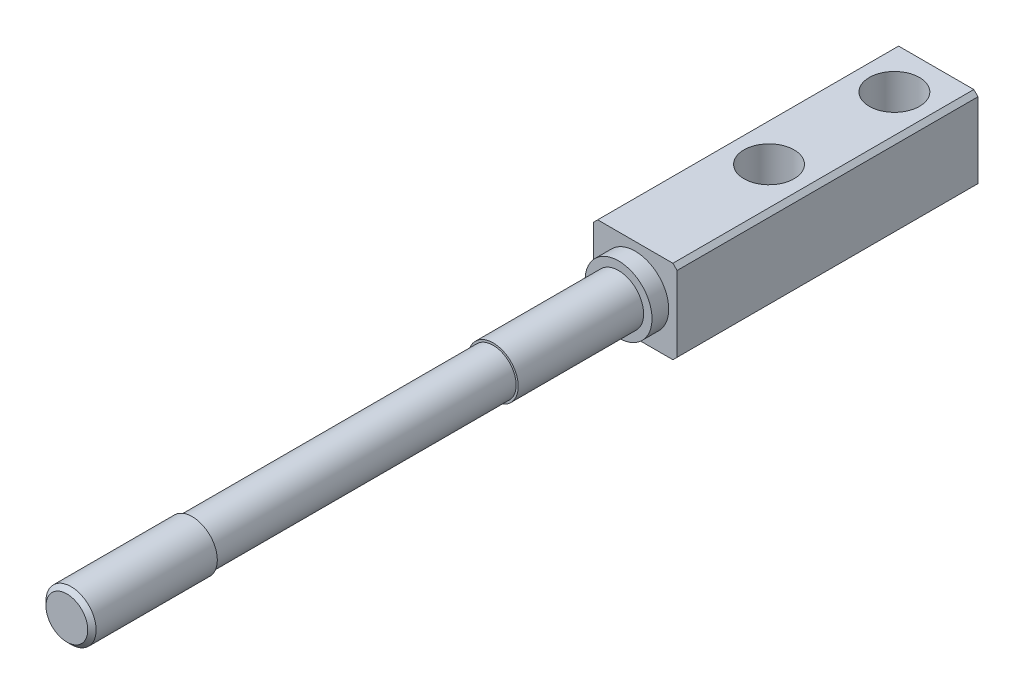
from build123d import *

# Parameters (mm, degrees)
SKETCH1_W           = 10
SKETCH1_H           = 10
BOSS_EXTRUDE1_DEPTH = 36
SKETCH2_R           = 4
BOSS_EXTRUDE2_DEPTH = 2
SKETCH3_R           = 3
BOSS_EXTRUDE3_DEPTH = 66
SKETCH4_R           = 3
CUT_EXTRUDE1_DEPTH  = 50
CHAMFER1_SIZE       = 0.5
CHAMFER2_SIZE       = 0.5
SKETCH6_W           = 5
SKETCH6_H           = 36


with BuildPart() as part:
    # Sketch1 → Boss-Extrude1 (new body)
    with BuildSketch(Plane.XY):
        Rectangle(SKETCH1_W, SKETCH1_H)
    extrude(amount=BOSS_EXTRUDE1_DEPTH)

    # Sketch2 → Boss-Extrude2 (add)
    with BuildSketch(Plane.XY.offset(36)):
        Circle(SKETCH2_R)
    extrude(amount=BOSS_EXTRUDE2_DEPTH)

    # Sketch3 → Boss-Extrude3 (add)
    with BuildSketch(Plane.XY.offset(38)):
        Circle(SKETCH3_R)
    extrude(amount=BOSS_EXTRUDE3_DEPTH)

    # Sketch4 → Cut-Extrude1 (cut)
    with BuildSketch(Plane(origin=(0, 5, 0), x_dir=(1, 0, 0), z_dir=(0, 1, 0))):
        with Locations(Location((0, -5, 0), (0, 0, 270))):
            Circle(SKETCH4_R)
        with Locations(Location((0, -20, 0), (0, 0, 270))):
            Circle(SKETCH4_R)
    extrude(amount=-CUT_EXTRUDE1_DEPTH, mode=Mode.SUBTRACT)

    # Chamfer1
    chamfer1_edges = [part.edges().sort_by_distance(p)[0] for p in [
        (5, -5, 18),
        (-5, -5, 18),
        (-5, 5, 18),
        (5, 5, 18),
    ]]
    chamfer(chamfer1_edges, length=CHAMFER1_SIZE)

    # Chamfer2
    chamfer2_edges = [part.edges().sort_by_distance(p)[0] for p in [
        (-3, 0, 104),
    ]]
    chamfer(chamfer2_edges, length=CHAMFER2_SIZE)

    # Sketch6 → Cut-Revolve1 (revolve, cut)
    with BuildSketch(Plane(origin=(0, 0, 0), x_dir=(1, 0, 0), z_dir=(0, 1, 0))):
        with Locations((5.25, -71)):
            Rectangle(SKETCH6_W, SKETCH6_H)
    revolve(axis=Axis((0, 0, 103.5), (0, 0, -1)), mode=Mode.SUBTRACT)


solid = part.part
